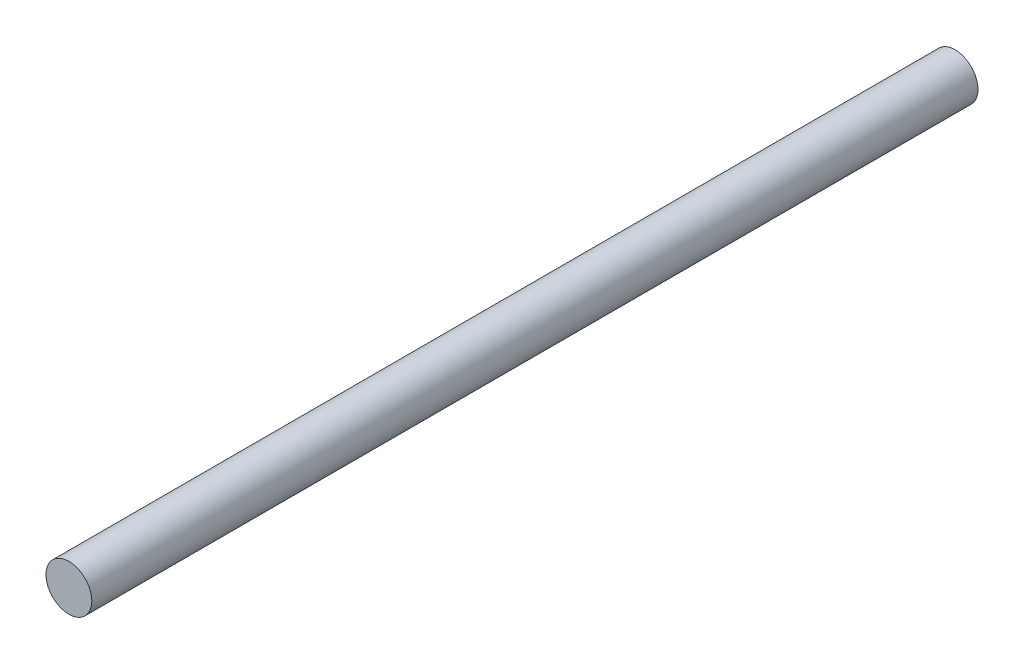
SolidWorks part; units mm, degrees
ref_plane "Front Plane" through (0, 0, 0) normal (0, 0, 1) x (1, 0, 0)
ref_plane "Top Plane" through (0, 0, 0) normal (0, 1, 0) x (1, 0, 0)
ref_plane "Right Plane" through (0, 0, 0) normal (1, 0, 0) x (0, 0, -1)
sketch "Sketch1" plane through (0, 0, 0) normal (0, 0, 1) x (1, 0, 0)
  circle A0 centre (0, 0) radius 4.5
  dimension "D1" = 9
extrude "Boss-Extrude1" add sketch "Sketch1" along normal blind 174
